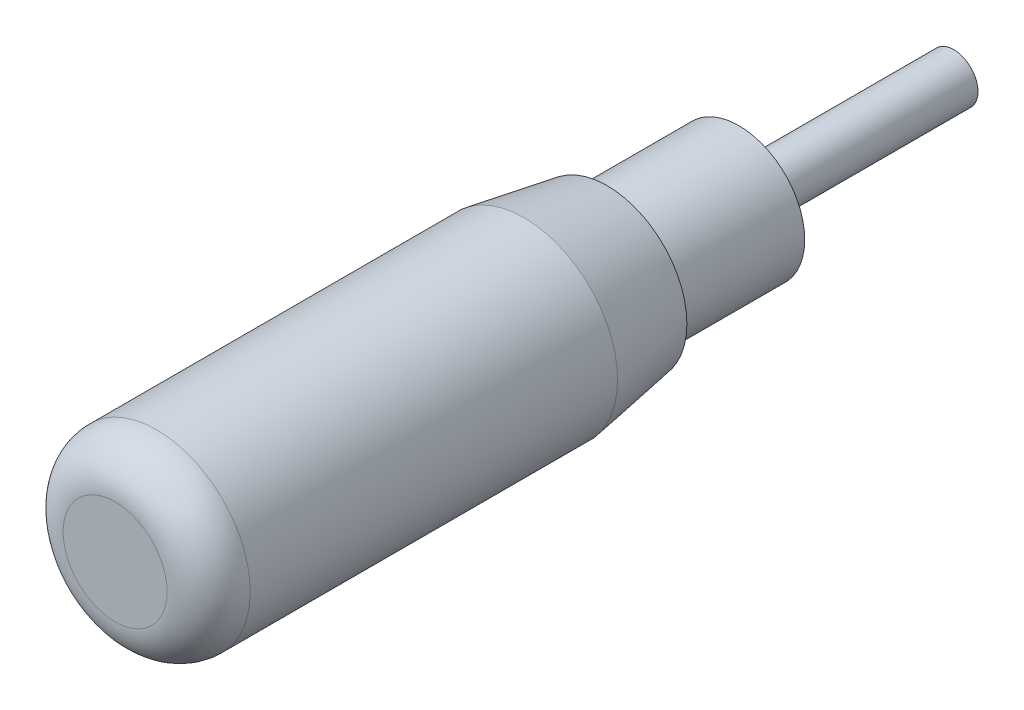
SolidWorks part; units mm, degrees
material "6061"
ref_plane "Front Plane" through (0, 0, 0) normal (0, 0, 1) x (1, 0, 0)
ref_plane "Top Plane" through (0, 0, 0) normal (0, 1, 0) x (1, 0, 0)
ref_plane "Right Plane" through (0, 0, 0) normal (1, 0, 0) x (0, 0, -1)
sketch "Sketch1" plane through (0, 0, 0) normal (0, 0, 1) x (1, 0, 0)
  circle A0 centre (0, 0) radius 1.75
  dimension "D1" = 3.5
extrude "Boss-Extrude1" add sketch "Sketch1" along normal blind 15.5
sketch "Sketch2" plane through (0, 0, 15.5) normal (0, 0, 1) x (1, 0, 0)
  circle A0 centre (0, 0) radius 4.75
  dimension "D1" = 9.5
extrude "Boss-Extrude2" add sketch "Sketch2" along normal blind 9.5
sketch "Sketch3" plane through (0, 0, 25) normal (0, 0, 1) x (1, 0, 0)
  circle A0 centre (0, 0) radius 6.75
  dimension "D1" = 13.5
extrude "Boss-Extrude3" add sketch "Sketch3" along normal blind 35.5
chamfer "Chamfer1" distance 1 distance2 6 1 edges at (6.75, 0, 25)
fillet "Fillet1" radius 3 1 edges at (6.75, 0, 60.5)
